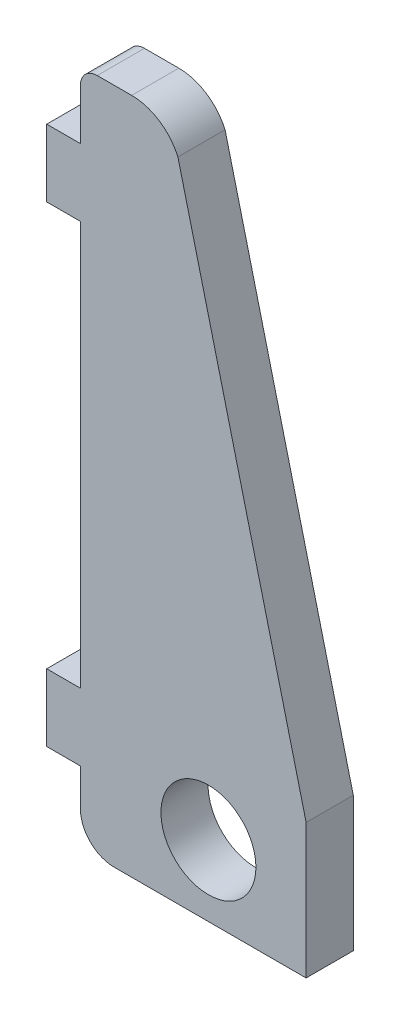
from build123d import *

# Parameters (mm, degrees)
SKETCH2_R           = 14.1
BOSS_EXTRUDE2_DEPTH = 14


with BuildPart() as part:
    # Sketch2 → Boss-Extrude2 (new body)
    with BuildSketch(Plane.XY):
        with BuildLine():
            Line((10, 181), (10, 196))
            ThreePointArc((10, 196), (11.464466094, 199.535533906), (15, 201))
            Line((15, 201), (25.209501406, 201))
            ThreePointArc((25.209501406, 201), (33.408153022, 198.561134968), (38.940750673, 192.037614891))
            Line((38.940750673, 192.037614891), (76.997541741, 40))
            Line((76.997541741, 40), (76.997541741, 30))
            Line((76.997541741, 30), (76.997541741, 10))
            Line((76.997541741, 10), (76.997541741, 0))
            Line((76.997541741, 0), (20, 0))
            ThreePointArc((20, 0), (12.928932188, 2.928932188), (10, 10))
            Line((10, 10), (10, 21))
            Line((10, 21), (0, 21))
            Line((0, 21), (0, 41))
            Line((0, 41), (10, 41))
            Line((10, 41), (10, 101))
            Line((10, 101), (10, 161))
            Line((10, 161), (0, 161))
            Line((0, 161), (0, 181))
            Line((0, 181), (10, 181))
        make_face()
        with Locations((48, 21)):
            Circle(SKETCH2_R, mode=Mode.SUBTRACT)
    extrude(amount=BOSS_EXTRUDE2_DEPTH)


solid = part.part
